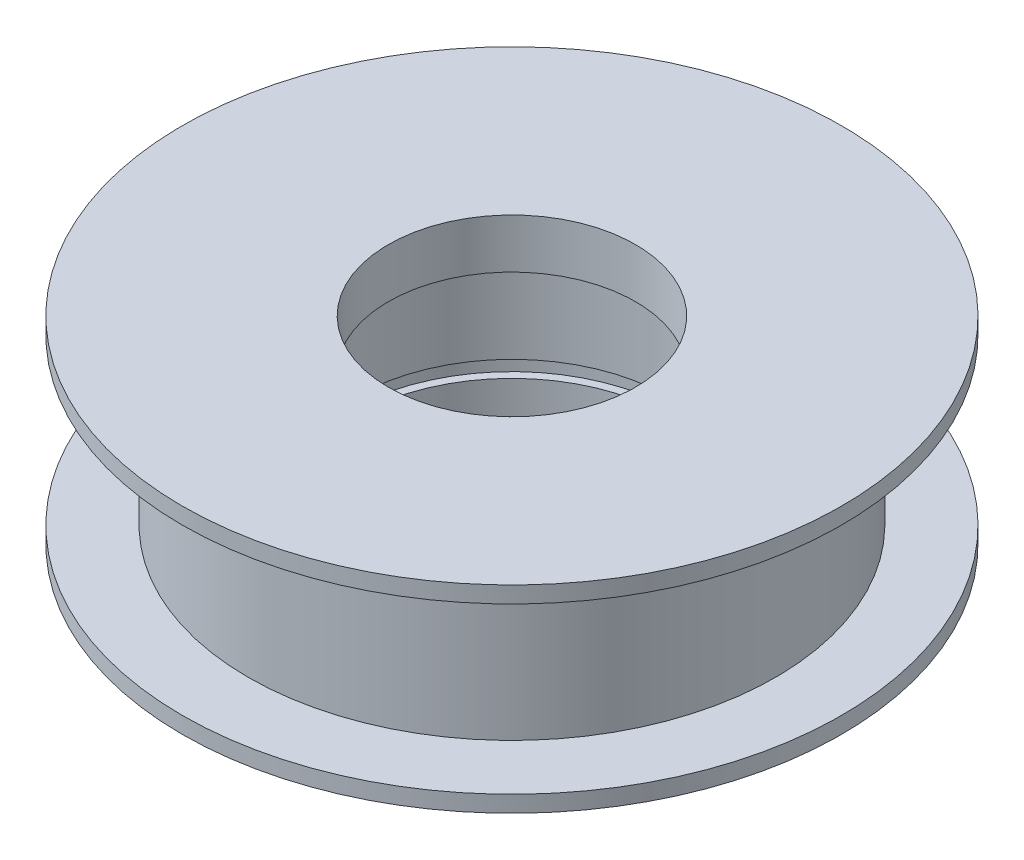
from build123d import *


with BuildPart() as part:
    # 草图1 → 旋转1 (revolve)
    with BuildSketch(Plane.XY, mode=Mode.PRIVATE) as revolve_1_sk:
        Polygon((7.5, 3), (7.5, 0), (9.5, 0), (9.5, -6), (10, -6), (10, -7), (9.5, -7), (9.5, -9), (20, -9), (20, -8), (16, -8), (16, 2), (20, 2), (20, 3), align=None)
    revolve(revolve_1_sk.sketch.rotate(Axis((0, 22.495377882, 0), (0, -1, 0)), 90), axis=Axis((0, 22.495377882, 0), (0, -1, 0)))


solid = part.part
